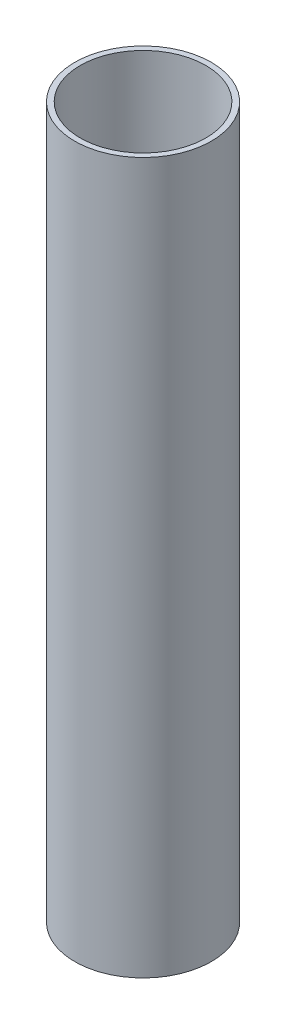
from build123d import *

# Parameters (mm, degrees)
SKETCH_1_R      = 2.5
SKETCH_1_R_2    = 2.3
EXTRUDE_1_DEPTH = 26


with BuildPart() as part:
    # 草图1 → 凸台-拉伸1 (new body)
    with BuildSketch(Plane(origin=(0, 0, 0), x_dir=(1, 0, 0), z_dir=(0, 1, 0))):
        with Locations(Location((0, 0, 0), (0, 0, 90))):
            Circle(SKETCH_1_R)
        with Locations(Location((0, 0, 0), (0, 0, 90))):
            Circle(SKETCH_1_R_2, mode=Mode.SUBTRACT)
    extrude(amount=EXTRUDE_1_DEPTH)


solid = part.part
